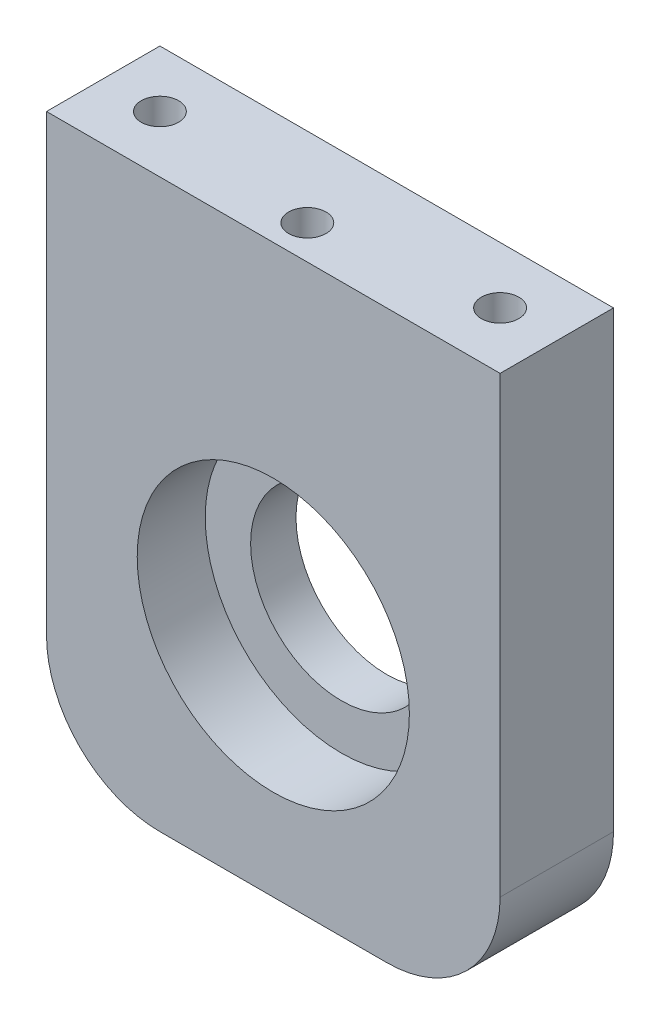
SolidWorks part; units mm, degrees
ref_plane "前视基准面" through (0, 0, 0) normal (0, 0, 1) x (1, 0, 0)
ref_plane "上视基准面" through (0, 0, 0) normal (0, 1, 0) x (1, 0, 0)
ref_plane "右视基准面" through (0, 0, 0) normal (1, 0, 0) x (0, 0, -1)
sketch "草图1" plane through (0, 0, 0) normal (0, 0, 1) x (1, 0, 0)
  line L1 (20, 25) -> (-20, 25)
  line L2 (20, 25) -> (20, -25)
  line L3 (20, -25) -> (-20, -25)
  line L4 (-20, 25) -> (-20, -25)
  line L5 (20, 25) -> (-20, -25) construction
  line L6 (20, -25) -> (-20, 25) construction
  point P0 (0, 0)
  dimension "D1" = 40
  dimension "D2" = 50
extrude "凸台-拉伸1" add sketch "草图1" along normal blind 10
sketch "草图2" plane through (0, 0, 10) normal (0, 0, 1) x (1, 0, 0)
  line L1 (20, 25) -> (-20, 25) construction
  circle A0 centre (0, -5) radius 12
  dimension "D1" = 24
  dimension "D2" = 30
extrude "切除-拉伸1" cut sketch "草图2" against normal blind 6
sketch "草图3" plane through (0, 0, 4) normal (0, 0, 1) x (1, 0, 0)
  line L1 (20, 25) -> (-20, 25) construction
  circle A0 centre (0, -5) radius 8
  dimension "D1" = 16
  dimension "D2" = 30
extrude "切除-拉伸2" cut sketch "草图3" against normal through all
hole_wizard "M4 螺纹孔1" positions "草图5" profile "草图4" tap size "M4" standard "Iso"
sketch "草图5" plane through (0, 25, 0) normal (0, 1, 0) x (1, 0, 0)
  line L0 (-20, -10) -> (-20, 0) construction
  line L1 (20, -10) -> (20, 0) construction
  point P0 (-15, -5)
  point P2 (15, -5)
  dimension "D1" = 5
  dimension "D2" = 5
sketch "草图4" plane through (-15, 25, 5) normal (1, 0, 0) x (0, 0, 1)
  line L0 (0, 0) -> (0, 10.9914)
  line L1 (0, 10.9914) -> (1.65, 10)
  line L2 (1.65, 10) -> (1.65, 0)
  line L5 (1.65, 0) -> (0, 0)
  line L10 (0, 10.9914) -> (-1.65, 10) construction
  line L11 (0, -6.35) -> (0, 107.95) construction
  dimension "螺纹孔钻头直径" = 3.3
  dimension "螺纹孔钻头深度" = 10
  dimension "导头角度" = 118
cosmetic thread "孔螺蚊线1" parameters "D1"=8, "D2"=4
cosmetic thread "孔螺蚊线2" parameters "D1"=8, "D2"=4
fillet "圆角1" radius 10 2 edges at (-20, -25, 5) (20, -25, 5)
hole_wizard "M4 螺纹孔3" positions "草图10" profile "草图11" tap size "M4" standard "Iso"
sketch "草图10" plane through (0, 25, 0) normal (0, 1, 0) x (1, 0, 0)
  line L0 (20, -10) -> (-20, -10) construction
  point P0 (0, -7)
  dimension "D1" = 3
sketch "草图11" plane through (0, 25, 7) normal (1, 0, 0) x (0, 0, 1)
  line L0 (0, 0) -> (0, 18)
  line L1 (0, 18) -> (1.65, 18)
  line L2 (1.65, 18) -> (1.65, 0)
  line L5 (1.65, 0) -> (0, 0)
  line L11 (0, -6.35) -> (0, 107.95) construction
  dimension "通孔螺纹孔钻头直径" = 3.3
  dimension "通孔螺纹孔钻头深度" = 18
cosmetic thread "孔螺蚊线4" parameters "D2"=4
